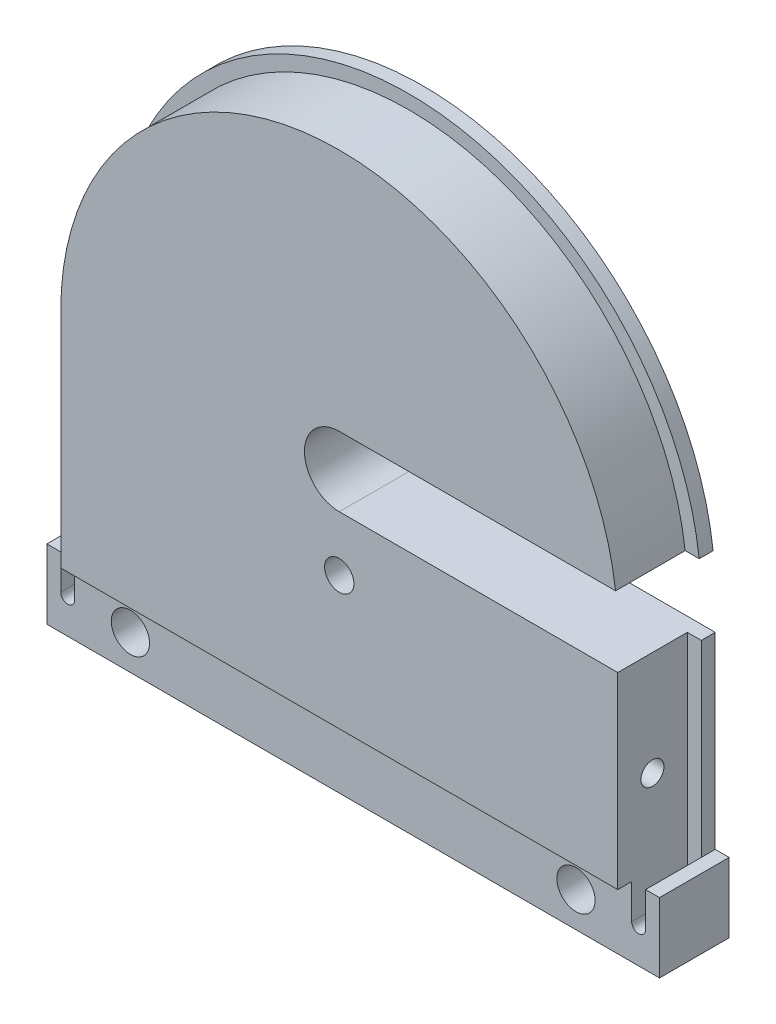
from build123d import *

# Parameters (mm, degrees)
EXTRUDE_1_DEPTH        = 12
CUT_EXTRUDE_START      = -10
CUT_EXTRUDE_1_DEPTH    = 10
SKETCH_3_W             = 2
SKETCH_3_H             = 10
CUT_EXTRUDE_2_DEPTH    = 109.889852603
CUT_EXTRUDE_3_DEPTH    = 8
CUT_EXTRUDE_4_DEPTH    = 78.775317421
SKETCH_6_R             = 2.75
CUT_EXTRUDE_5_DEPTH    = 78.775317421
SKETCH_7_R             = 4.5
CUT_EXTRUDE_6_DEPTH    = 6
HOLE_WIZARD_M4_1_D     = 3.3
HOLE_WIZARD_M4_1_DEPTH = 10
HOLE_WIZARD_M4_1_TIP   = 0.991420021
HOLE_WIZARD_M4_2_D     = 3.3
HOLE_WIZARD_M4_2_DEPTH = 10
HOLE_WIZARD_M4_2_TIP   = 0.991420021
HOLE_WIZARD_M5_1_D     = 4.2


with BuildPart() as part:
    # 草图1 → 凸台-拉伸1 (new body)
    with BuildSketch(Plane.XY):
        with BuildLine():
            Line((-44, -11), (-44, -21))
            Line((-44, -21), (44, -21))
            Line((44, -21), (44, -11))
            Line((44, -11), (42, -11))
            Line((42, -11), (42, 21))
            ThreePointArc((42, 21), (0, 63), (-42, 21))
            Line((-42, 21), (-42, -11))
            Line((-42, -11), (-44, -11))
        make_face()
    extrude(amount=EXTRUDE_1_DEPTH)

    # 草图2 → 切除-拉伸1 (cut)
    with BuildSketch(Plane.XY.offset(12).offset(CUT_EXTRUDE_START)):
        with BuildLine():
            Line((-40, 21), (-40, -11))
            Line((-40, -11), (-42, -11))
            Line((-42, -11), (-42, 21))
            ThreePointArc((-42, 21), (0, 63), (42, 21))
            Line((42, 21), (42, -11))
            Line((42, -11), (40, -11))
            Line((40, -11), (40, 21))
            ThreePointArc((40, 21), (0, 61), (-40, 21))
        make_face()
    extrude(amount=CUT_EXTRUDE_1_DEPTH, mode=Mode.SUBTRACT)

    # 草图3 → 切除-拉伸2 (cut, through all)
    with BuildSketch(Plane(origin=(44, 0, 0), x_dir=(0, 0, -1), z_dir=(1, 0, 0))):
        with Locations((-11, -16)):
            Rectangle(SKETCH_3_W, SKETCH_3_H)
    extrude(amount=-CUT_EXTRUDE_2_DEPTH, mode=Mode.SUBTRACT)

    # 草图4 → 切除-拉伸3 (cut)
    with BuildSketch(Plane.XY.offset(10)):
        with BuildLine():
            Line((-40, -11), (-42, -11))
            Line((-42, -11), (-42, -16))
            ThreePointArc((-42, -16), (-41, -17), (-40, -16))
            Line((-40, -16), (-40, -11))
        make_face()
        with BuildLine():
            Line((42, -11), (42, -16))
            ThreePointArc((42, -16), (41, -17), (40, -16))
            Line((40, -16), (40, -11))
            Line((40, -11), (42, -11))
        make_face()
    extrude(amount=-CUT_EXTRUDE_3_DEPTH, mode=Mode.SUBTRACT)

    # 草图5 → 切除-拉伸4 (cut, through all)
    with BuildSketch(Plane(origin=(0, 0, 0), x_dir=(-1, 0, 0), z_dir=(0, 0, -1))):
        with BuildLine():
            Line((0, 26), (-46.263882953, 26))
            Line((-46.263882953, 26), (-46.263882953, 16))
            Line((-46.263882953, 16), (0, 16))
            ThreePointArc((0, 16), (5, 21), (0, 26))
        make_face()
    extrude(amount=-CUT_EXTRUDE_4_DEPTH, mode=Mode.SUBTRACT)

    # 草图6 → 切除-拉伸5 (cut, through all)
    with BuildSketch(Plane(origin=(0, 0, 0), x_dir=(-1, 0, 0), z_dir=(0, 0, -1))):
        with Locations((-32, -16)):
            Circle(SKETCH_6_R)
        with Locations((32, -16)):
            Circle(SKETCH_6_R)
    extrude(amount=-CUT_EXTRUDE_5_DEPTH, mode=Mode.SUBTRACT)

    # 草图7 → 切除-拉伸6 (cut)
    with BuildSketch(Plane(origin=(0, 0, 0), x_dir=(-1, 0, 0), z_dir=(0, 0, -1))):
        with Locations((-32, -16)):
            Circle(SKETCH_7_R)
        with Locations((32, -16)):
            Circle(SKETCH_7_R)
    extrude(amount=-CUT_EXTRUDE_6_DEPTH, mode=Mode.SUBTRACT)

    # M4 螺纹孔1
    with Locations(Plane(origin=(-40, 1, 7), x_dir=(0, 0, -1), z_dir=(-1, 0, 0))):
        with Locations((0, 0)):
            Hole(HOLE_WIZARD_M4_1_D / 2, depth=HOLE_WIZARD_M4_1_DEPTH)
            with Locations((0, 0, -(HOLE_WIZARD_M4_1_DEPTH + HOLE_WIZARD_M4_1_TIP / 2))):  # 118° drill point
                Cone(0, HOLE_WIZARD_M4_1_D / 2, HOLE_WIZARD_M4_1_TIP, mode=Mode.SUBTRACT)

    # M4 螺纹孔2
    with Locations(Plane(origin=(40, 1, 7.015407491), x_dir=(0, 0, 1), z_dir=(1, 0, 0))):
        with Locations((0, 0)):
            Hole(HOLE_WIZARD_M4_2_D / 2, depth=HOLE_WIZARD_M4_2_DEPTH)
            with Locations((0, 0, -(HOLE_WIZARD_M4_2_DEPTH + HOLE_WIZARD_M4_2_TIP / 2))):  # 118° drill point
                Cone(0, HOLE_WIZARD_M4_2_D / 2, HOLE_WIZARD_M4_2_TIP, mode=Mode.SUBTRACT)

    # M5 螺纹孔1 (through all)
    with Locations(Plane(origin=(0, 8.081866722, 0), x_dir=(-1, 0, 0), z_dir=(0, 0, -1))):
        with Locations((0, 0)):
            Hole(HOLE_WIZARD_M5_1_D / 2)


solid = part.part
